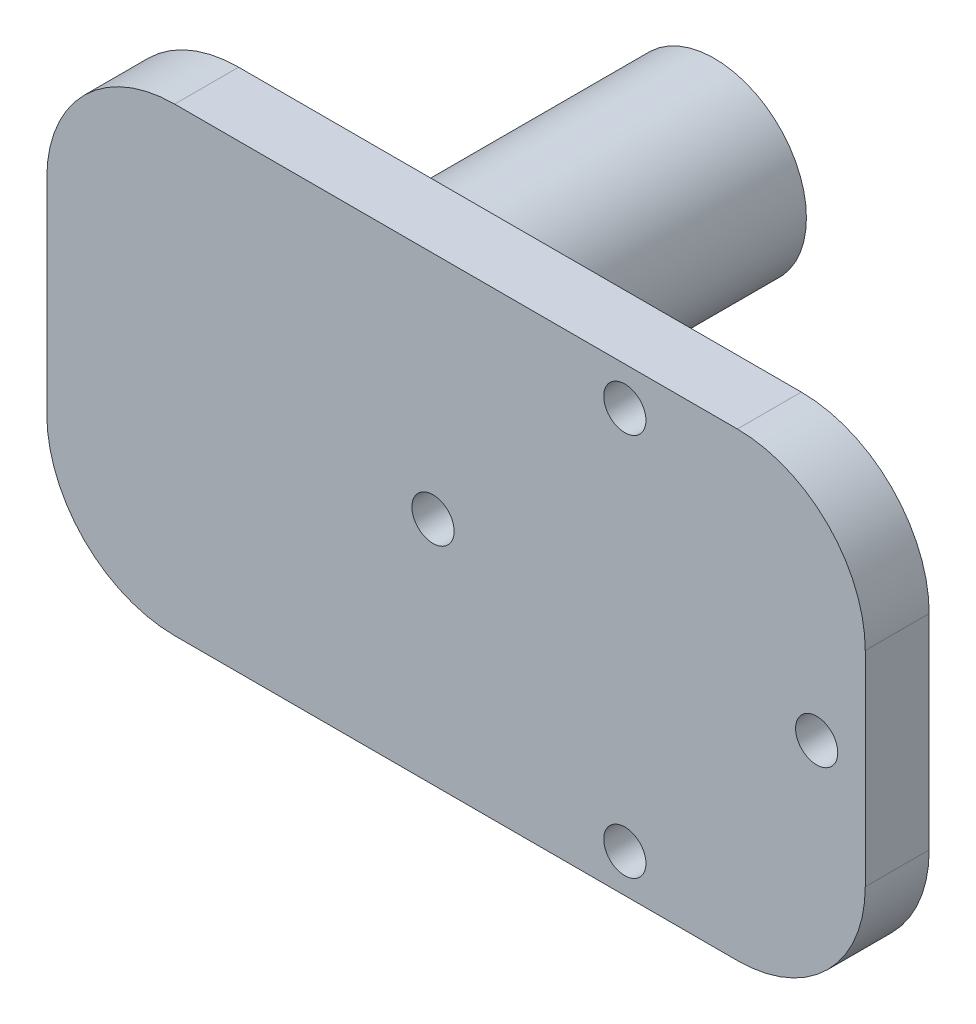
SolidWorks part; units mm, degrees
ref_plane "前视基准面" through (0, 0, 0) normal (0, 0, 1) x (1, 0, 0)
ref_plane "上视基准面" through (0, 0, 0) normal (0, 1, 0) x (1, 0, 0)
ref_plane "右视基准面" through (0, 0, 0) normal (1, 0, 0) x (0, 0, -1)
sketch "草图1" plane through (0, 0, 0) normal (0, 0, 1) x (1, 0, 0)
  circle A0 centre (0, 0) radius 7.2
  circle A1 centre (0, 0) radius 4.2
  dimension "D1" = 8.4
  dimension "D2" = 3
extrude "凸台-拉伸1" add sketch "草图1" along normal mid plane 15
sketch "草图2" plane through (0, 0, 7.5) normal (0, 0, 1) x (1, 0, 0)
  circle A0 centre (0, 0) radius 7.2 construction
  circle A1 centre (0, 0) radius 7.2
extrude "凸台-拉伸2" add sketch "草图2" along normal blind 20
sketch "草图3" plane through (0, 0, 27.5) normal (0, 0, 1) x (1, 0, 0)
  line L0 (0, 0) -> (0, 7.2) construction
  line L1 (0, 7.2) -> (0, 17.2) construction
  circle A0 centre (0, 0) radius 17.2
  circle A1 centre (0, 0) radius 7.2 construction
  circle A3 centre (0, 0) radius 7.2
  dimension "D1" = 10
extrude "凸台-拉伸3" add sketch "草图3" against normal blind 3
sketch "草图4" plane through (0, 0, 24.5) normal (0, 0, -1) x (-1, 0, 0)
  line L1 (0, 13.35) -> (0, 15) construction
  line L2 (0, 15) -> (0, 17.2) construction
  circle A1 centre (0, 0) radius 17.2 construction
  circle A2 centre (0, 15) radius 1.65
  dimension "D1" = 3.3
  dimension "D2" = 15
extrude "切除-拉伸1" cut sketch "草图4" against normal blind 3
pattern_circular "阵列(圆周)1" count 4 over 360 about axis through (0, 0, 0) along (0, 0, 1) of "切除-拉伸1"
sketch "草图5" plane through (0, 0, 27.5) normal (0, 0, 1) x (1, 0, 0)
  line L0 (0, 0) -> (14.8, 0) construction
  line L1 (46.8, -18) -> (-17.2, -18)
  line L2 (46.8, -18) -> (46.8, 18)
  line L3 (46.8, 18) -> (-17.2, 18)
  line L4 (-17.2, -18) -> (-17.2, 18)
  line L5 (46.8, -18) -> (-17.2, 18) construction
  line L6 (46.8, 18) -> (-17.2, -18) construction
  circle A0 centre (0, 0) radius 17.2 construction
  point P0 (14.8, 0)
  dimension "D1" = 64
  dimension "D2" = 36
extrude "凸台-拉伸4" add sketch "草图5" against normal blind 5
sketch "草图6" plane through (0, 0, 27.5) normal (0, 0, 1) x (1, 0, 0)
  line L0 (0, 0) -> (28, 0) construction
  line L1 (28, 15) -> (28, 0) construction
  circle A0 centre (28, 0) radius 15 construction
  circle A1 centre (28, 15) radius 1.65
  circle A2 centre (43, 0) radius 1.65
  circle A3 centre (28, -15) radius 1.65
  circle A4 centre (13, 0) radius 1.65
  point P15 (28, 0)
  dimension "D1" = 30
  dimension "D3" = 3.3
  dimension "D2" = 28
  dimension "D4" = 4
extrude "切除-拉伸2" cut sketch "草图6" against normal blind 50
fillet "圆角1" radius 10 4 edges at (-17.2, 18, 25) (-17.2, -18, 25) (46.8, -18, 25) (46.8, 18, 25)
sketch "草图7" plane through (0, 0, 7.5) normal (0, 0, -1) x (-1, 0, 0)
  circle A1 centre (0, 0) radius 4.2
  circle A2 centre (0, 0) radius 4.2
  dimension "D1" = 0
extrude "切除-拉伸3" cut sketch "草图7" against normal blind 10
